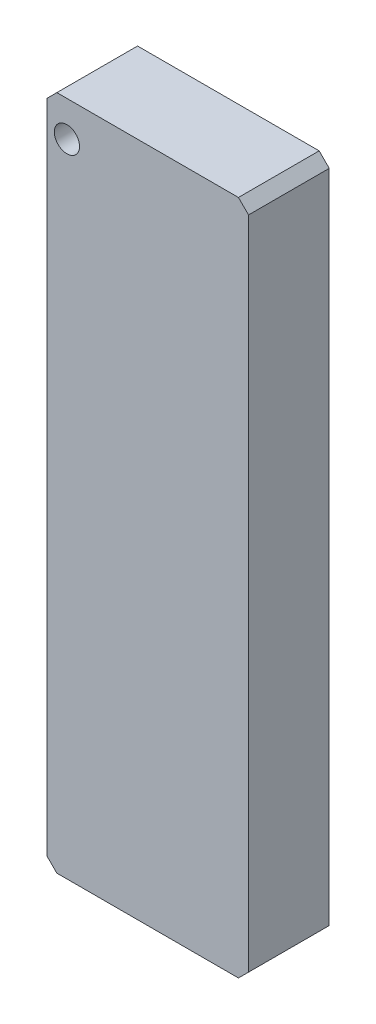
SolidWorks part; units mm, degrees
material "A6061"
ref_plane "前基準面" through (0, 0, 0) normal (0, 0, 1) x (1, 0, 0)
ref_plane "上基準面" through (0, 0, 0) normal (0, 1, 0) x (1, 0, 0)
ref_plane "右基準面" through (0, 0, 0) normal (1, 0, 0) x (0, 0, -1)
sketch "草图1" plane through (0, 0, 0) normal (0, 0, 1) x (1, 0, 0)
  line L1 (-10, 33.5) -> (10, 33.5)
  line L2 (-10, 33.5) -> (-10, -33.5)
  line L3 (-10, -33.5) -> (10, -33.5)
  line L4 (10, 33.5) -> (10, -33.5)
  line L5 (-10, 33.5) -> (10, -33.5) construction
  line L6 (-10, -33.5) -> (10, 33.5) construction
  point P0 (0, 0)
  dimension "D1" = 67
  dimension "D2" = 20
extrude "凸台-拉伸1" add sketch "草图1" along normal mid plane 8
sketch "草图3" plane through (0, 0, -4) normal (0, 0, -1) x (-1, 0, 0)
  line L3 (-10, 33.5) -> (10, 33.5) construction
  line L4 (10, 33.5) -> (10, -33.5) construction
  point P0 (8, 30)
  dimension "D1" = 3.5
  dimension "D2" = 2
hole_wizard "M3 螺纹孔1" positions "草图3" profile "草图4" tap size "M3" standard "GB" end condition through all
sketch "草图4" plane through (-8, 30, -4) normal (1, 0, 0) x (0, 1, 0)
  line L0 (0, 0) -> (0, 8)
  line L1 (0, 8) -> (1.25, 8)
  line L2 (1.25, 8) -> (1.25, 0)
  line L5 (1.25, 0) -> (0, 0)
  line L11 (0, -6.35) -> (0, 107.95) construction
  dimension "通孔螺纹孔钻头直径" = 2.5
  dimension "通孔螺纹孔钻头深度" = 8
cosmetic thread "孔螺蚊线1" parameters "D2"=3
sketch "草图8" plane through (0, -33.5, 0) normal (0, -1, 0) x (-1, 0, 0)
  line L0 (0, 1.8637) -> (0, -2.6969) construction
  point P0 (6, 0)
  point P8 (-6, 0)
  dimension "D1" = 12
hole_wizard "M4 螺纹孔1" positions "草图8" profile "草图9" tap size "M4" standard "GB"
sketch "草图9" plane through (-6, -33.5, 0) normal (1, 0, 0) x (0, 0, -1)
  line L0 (0, 0) -> (0, 11.0914)
  line L1 (0, 11.0914) -> (1.65, 10.1)
  line L2 (1.65, 10.1) -> (1.65, 0)
  line L5 (1.65, 0) -> (0, 0)
  line L10 (0, 11.0914) -> (-1.65, 10.1) construction
  line L11 (0, -6.35) -> (0, 107.95) construction
  dimension "螺纹孔钻头直径" = 3.3
  dimension "螺纹孔钻头深度" = 10.1
  dimension "导头角度" = 118
cosmetic thread "孔螺蚊线2" parameters "D1"=8, "D2"=4
cosmetic thread "孔螺蚊线3" parameters "D1"=8, "D2"=4
chamfer "倒角1" distance 1 angle 45 4 edges at (-10, -33.5, 0) (10, -33.5, 0) (10, 33.5, 0) (-10, 33.5, 0)
